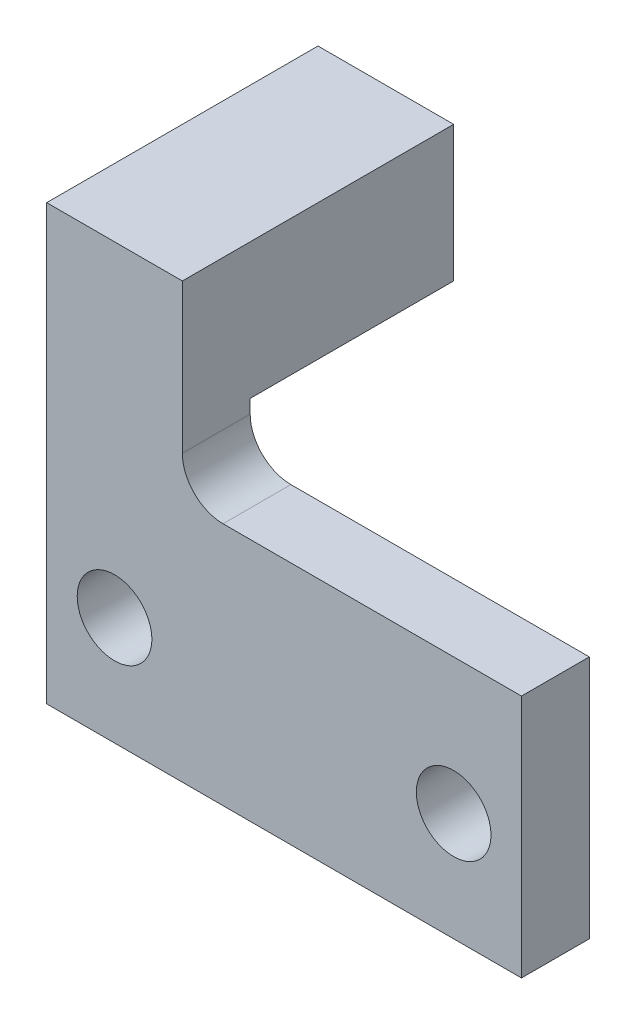
SolidWorks part; units mm, degrees
ref_plane "前视基准面" through (0, 0, 0) normal (0, 0, 1) x (1, 0, 0)
ref_plane "上视基准面" through (0, 0, 0) normal (0, 1, 0) x (1, 0, 0)
ref_plane "右视基准面" through (0, 0, 0) normal (1, 0, 0) x (0, 0, -1)
sketch "草图1" plane through (0, 0, 0) normal (0, 0, 1) x (1, 0, 0)
  line L1 (0, 0) -> (35, 0)
  line L2 (0, 0) -> (0, 22)
  line L3 (13, 18) -> (35, 18)
  line L4 (35, 0) -> (35, 18)
  line L7 (0, 22) -> (10, 22)
  line L8 (10, 21) -> (10, 22)
  arc A0 (13, 18) -> (10, 21) centre (13, 21) cw
  dimension "D4" = 3
  dimension "D1" = 18
  dimension "D2" = 35
  dimension "D3" = 22
  dimension "D5" = 10
  dimension "D6" = 1
extrude "凸台-拉伸1" add sketch "草图1" along normal blind 5
sketch "草图3" plane through (0, 0, 5) normal (0, 0, 1) x (1, 0, 0)
  line L1 (0, 22) -> (10, 22)
  line L2 (0, 22) -> (0, 32)
  line L3 (0, 32) -> (10, 32)
  line L4 (10, 22) -> (10, 32)
  dimension "D1" = 10
  dimension "D2" = 10
extrude "凸台-拉伸2" add sketch "草图3" against normal blind 20
sketch "草图4" plane through (0, 0, 0) normal (0, 0, -1) x (-1, 0, 0)
  line L0 (-10, 32) -> (0, 32) construction
  line L1 (-17.5, 0) -> (-17.5, 27.8202) construction
  line L2 (0, 0) -> (-35, 0) construction
  circle A0 centre (-30, 8) radius 2.75
  circle A1 centre (-5, 8) radius 2.75
  dimension "D3" = 25
  dimension "D5" = 5.5
  dimension "D6" = 5.5
  dimension "D1" = 24
  dimension "D2" = 24
  dimension "D4" = 12.5
extrude "切除-拉伸1" cut sketch "草图4" against normal blind 20
